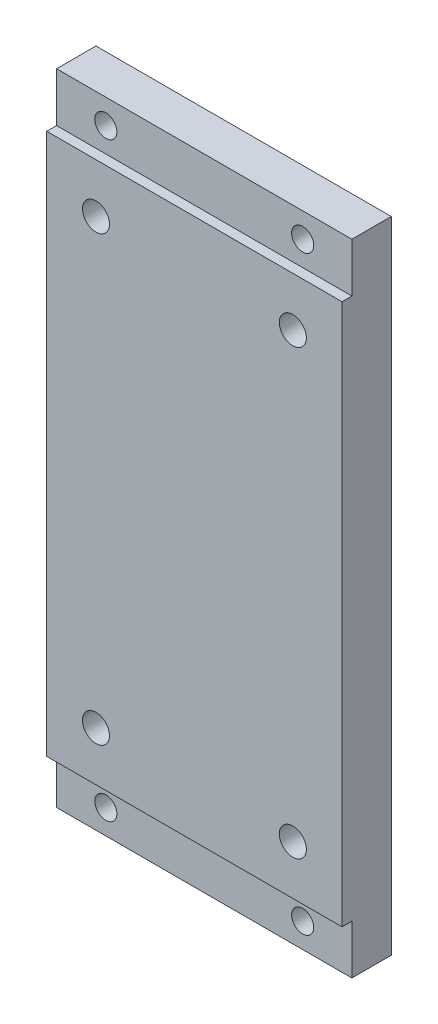
from build123d import *

# Parameters (mm, degrees)
SKETCH1_W                                           = 60
SKETCH1_H                                           = 130
BOSS_EXTRUDE1_DEPTH                                 = 10
SKETCH2_W                                           = 60
SKETCH2_H                                           = 10
CUT_EXTRUDE1_DEPTH                                  = 2
HOLE_SIZE_BY_SOCKET_HEAD_CAP_SCREW_TYPE_D           = 4.5
HOLE_SIZE_BY_SOCKET_HEAD_CAP_SCREW_TYPE_CBORE_D     = 8
HOLE_SIZE_BY_SOCKET_HEAD_CAP_SCREW_TYPE_CBORE_DEPTH = 4.6
M5_CLEARANCE_HOLE1_D                                = 5.5
M5_CLEARANCE_HOLE1_DEPTH                            = 15
M5_CLEARANCE_HOLE1_TIP                              = 1.652366702


with BuildPart() as part:
    # Sketch1 → Boss-Extrude1 (new body)
    with BuildSketch(Plane.XY):
        Rectangle(SKETCH1_W, SKETCH1_H)
    extrude(amount=BOSS_EXTRUDE1_DEPTH)

    # Sketch2 → Cut-Extrude1 (cut)
    with BuildSketch(Plane.XY.offset(10)):
        with Locations((0, 60)):
            Rectangle(SKETCH2_W, SKETCH2_H)
        with Locations((0, -60)):
            Rectangle(SKETCH2_W, SKETCH2_H)
    extrude(amount=-CUT_EXTRUDE1_DEPTH, mode=Mode.SUBTRACT)

    # Hole Size by Socket Head Cap Screw Type 1 (through all)
    with Locations(Plane(origin=(0, 0, 0), x_dir=(-1, 0, 0), z_dir=(0, 0, -1))):
        with Locations((20, -60), (-20, -60), (20, 60), (-20, 60)):
            CounterBoreHole(HOLE_SIZE_BY_SOCKET_HEAD_CAP_SCREW_TYPE_D / 2, HOLE_SIZE_BY_SOCKET_HEAD_CAP_SCREW_TYPE_CBORE_D / 2, HOLE_SIZE_BY_SOCKET_HEAD_CAP_SCREW_TYPE_CBORE_DEPTH)

    # M5 Clearance Hole1
    with Locations(Plane.XY.offset(10)):
        with Locations((-20, -45), (20, 45), (20, -45), (-20, 45)):
            Hole(M5_CLEARANCE_HOLE1_D / 2, depth=M5_CLEARANCE_HOLE1_DEPTH)
            with Locations((0, 0, -(M5_CLEARANCE_HOLE1_DEPTH + M5_CLEARANCE_HOLE1_TIP / 2))):  # 118° drill point
                Cone(0, M5_CLEARANCE_HOLE1_D / 2, M5_CLEARANCE_HOLE1_TIP, mode=Mode.SUBTRACT)


solid = part.part
